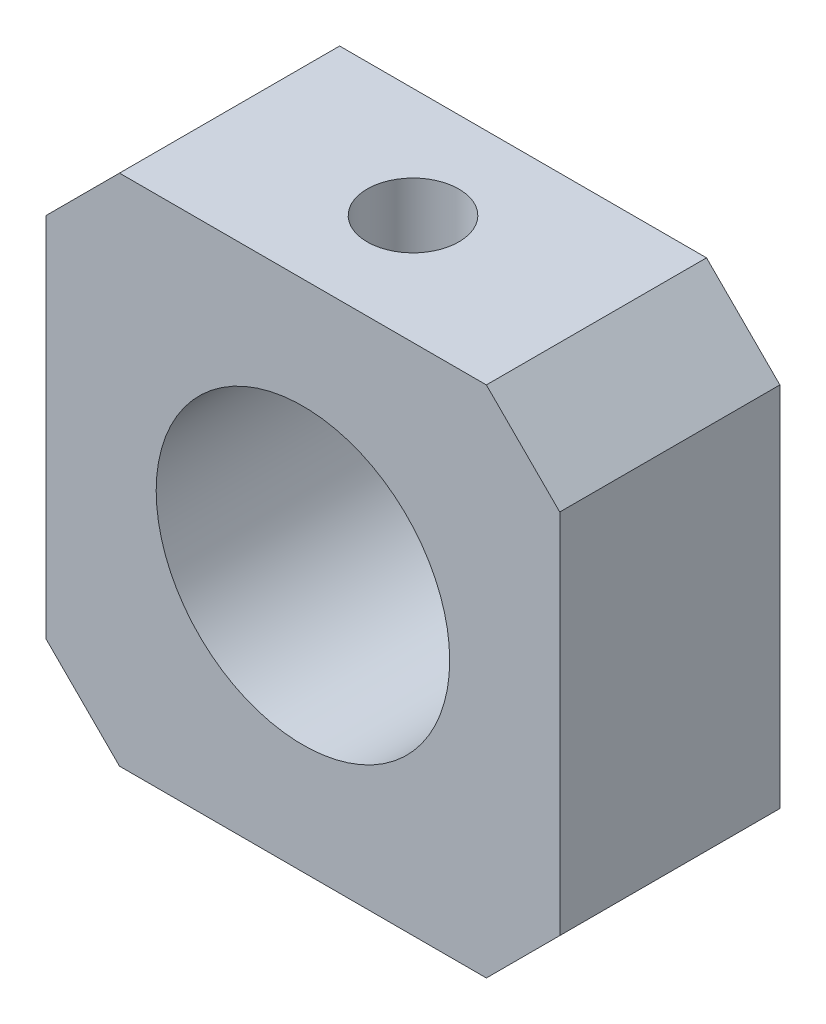
SolidWorks part; units mm, degrees
ref_plane "前视基准面" through (0, 0, 0) normal (0, 0, 1) x (1, 0, 0)
ref_plane "上视基准面" through (0, 0, 0) normal (0, 1, 0) x (1, 0, 0)
ref_plane "右视基准面" through (0, 0, 0) normal (1, 0, 0) x (0, 0, -1)
sketch "草图1" plane through (0, 0, 0) normal (0, 0, 1) x (1, 0, 0)
  line L1 (-7, -7) -> (7, -7)
  line L2 (-7, -7) -> (-7, 7)
  line L3 (-7, 7) -> (7, 7)
  line L4 (7, -7) -> (7, 7)
  line L5 (-7, -7) -> (7, 7) construction
  line L6 (-7, 7) -> (7, -7) construction
  circle A0 centre (0, 0) radius 4
  point P0 (0, 0)
  dimension "D1" = 8
  dimension "D2" = 14
extrude "凸台-拉伸1" add sketch "草图1" along normal mid plane 6
hole_wizard "M3 螺纹孔1" positions "3D草图1" profile "草图2" tap size "M3" standard "GB"
sketch3d "3D草图1"
  line L0 (0, 7, -3) -> (0, 7, 3)
  line L1 (7, 7, -3) -> (-7, 7, -3) construction
  line L2 (7, 7, 3) -> (-7, 7, 3) construction
  point P0 (0, 7, 0)
sketch "草图2" plane through (0, 7, 0) normal (1, 0, 0) x (0, 0, 1)
  line L0 (0, 0) -> (0, 3)
  line L1 (0, 3) -> (1.25, 3)
  line L2 (1.25, 3) -> (1.25, 0)
  line L5 (1.25, 0) -> (0, 0)
  line L11 (0, -6.35) -> (0, 107.95) construction
  dimension "通孔螺纹孔钻头直径" = 2.5
  dimension "通孔螺纹孔钻头深度" = 3
cosmetic thread "孔螺蚊线1"
chamfer "倒角2" distance 2 angle 45 4 edges at (-7, -7, 0) (7, -7, 0) (7, 7, 0) (-7, 7, 0)
